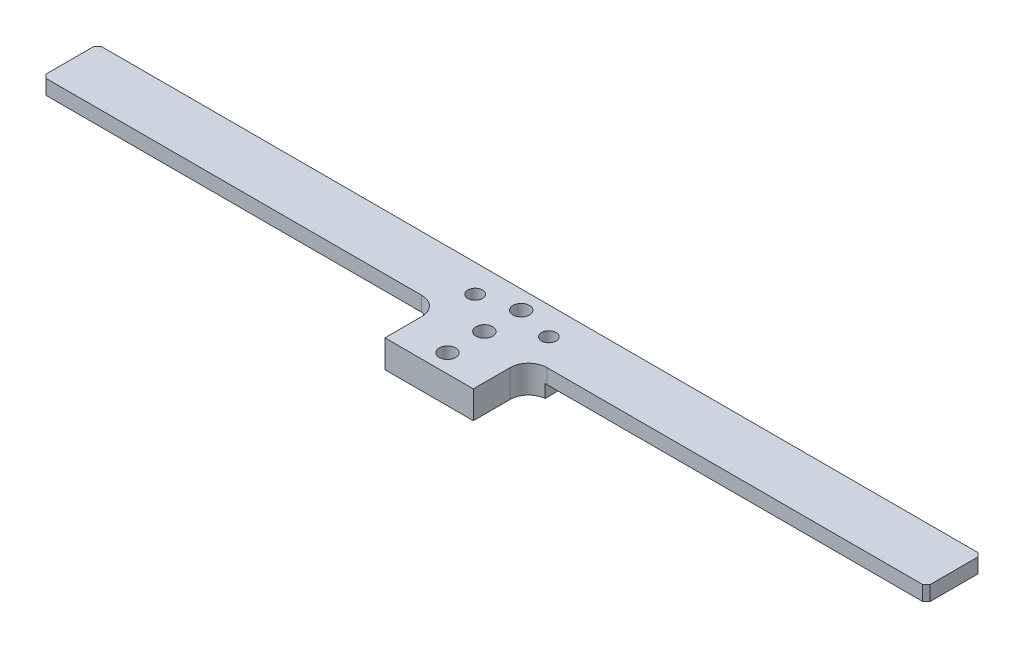
SolidWorks part; units mm, degrees
ref_plane "Front Plane" through (0, 0, 0) normal (0, 0, 1) x (1, 0, 0)
ref_plane "Top Plane" through (0, 0, 0) normal (0, 1, 0) x (1, 0, 0)
ref_plane "Right Plane" through (0, 0, 0) normal (1, 0, 0) x (0, 0, -1)
ref_plane "Plane 4" through (0, -2, 0) normal (0, -1, 0) x (1, 0, 0)
sketch "Sketch 1" plane through (0, -2, 0) normal (0, -1, 0) x (1, 0, 0)
  line L0 (-59, 15) -> (-69, 15)
  line L1 (-59, 15) -> (-58, 15)
  line L2 (-70, 15) -> (-70, -15)
  line L4 (-69, -15) -> (69, -15)
  line L5 (69, -15) -> (70, -14)
  line L6 (70, -14) -> (70, -1)
  line L7 (70, -1) -> (69, 0)
  line L8 (69, 0) -> (-53, 0)
  line L9 (-58, 5) -> (-58, 15)
  line L11 (-69, -15) -> (-70, -15)
  line L12 (-69, 15) -> (-70, 15)
  arc A3 (-53, 0) -> (-58, 5) centre (-53, 5) cw
  dimension "D1" = 5
extrude "Boss-Extrude 1" add sketch "Sketch 1" against normal blind 4
sketch "Sketch 2" plane through (0, 2, 0) normal (0, 1, 0) x (1, 0, 0)
  line L1 (-70, 15) -> (-190, 15)
  line L2 (-70, 15) -> (-70, -15)
  line L3 (-70, -15) -> (-82, -15)
  line L4 (-190, 15) -> (-190, 0)
  line L8 (-190, 0) -> (-82, 0)
  line L9 (-82, -15) -> (-82, 0)
  dimension "D1" = 120
  dimension "D2" = 12
  dimension "D3" = 15
extrude "Boss-Extrude 2" add sketch "Sketch 2" against normal blind 4
fillet "Fillet 1" radius 5 1 edges at (-82, 0, 0)
sketch "Sketch 6" plane through (0, -2, 0) normal (0, -1, 0) x (1, 0, 0)
  line L0 (-190, -15) -> (69, -15) construction
  line L1 (-82, 15) -> (-58, 15)
  line L2 (-82, 15) -> (-82, -15)
  line L3 (-82, -15) -> (-58, -15)
  line L4 (-58, 15) -> (-58, -15)
  dimension "D1" = 24
extrude "Boss-Extrude 3" add sketch "Sketch 6" along normal blind 3.5
sketch "Sketch 3" plane through (0, 2, 0) normal (0, 1, 0) x (1, 0, 0)
  line L0 (-82, -5) -> (-82, -15) construction
  line L2 (-58, -15) -> (-82, -15) construction
  circle A0 centre (-70, -10) radius 2.25
  dimension "D1" = 4.5
  dimension "D2" = 12
  dimension "D3" = 5
extrude "Cut-Extrude 1" cut sketch "Sketch 3" against normal through all
pattern_linear "Linear Pattern 1" count 3 spacing 10 along (0, 0, -1) of "Cut-Extrude 1"
sketch "Sketch 7" plane through (0, 2, 0) normal (0, 1, 0) x (1, 0, 0)
  line L0 (-58, -15) -> (-82, -15) construction
  line L1 (113.7784, -21.1495) -> (50, -21.1495)
  line L2 (113.7784, -21.1495) -> (113.7784, 35.093)
  line L3 (113.7784, 35.093) -> (50, 35.093)
  line L4 (50, -21.1495) -> (50, 35.093)
  point P6 (-70, -15)
  dimension "D1" = 120
extrude "Cut-Extrude 2" cut sketch "Sketch 7" against normal blind 10
chamfer "Chamfer 3" distance 1 angle 45 4 edges at (50, 0, -15) (50, 0, 0) (-190, 0, -15) (-190, 0, 0)
sketch "Sketch 8" plane through (0, -5.5, 0) normal (0, -1, 0) x (1, 0, 0)
  line L1 (-58, -15) -> (-53.5, -15)
  line L2 (-58, -15) -> (-58, 15)
  line L3 (-58, 15) -> (-53.5, 15)
  line L4 (-53.5, -15) -> (-53.5, 15)
  line L5 (-82, -15) -> (-86.5, -15)
  line L6 (-82, -15) -> (-82, 15)
  line L7 (-82, 15) -> (-86.5, 15)
  line L8 (-86.5, -15) -> (-86.5, 15)
  dimension "D1" = 30
  dimension "D2" = 4.5
  dimension "D3" = 4.5
  dimension "D4" = 30
extrude "Boss-Extrude 4" add sketch "Sketch 8" against normal up to surface (3.5 mm away) up to face at (-3.1429, -2, -7.5)
sketch "Sketch 9" plane through (0, -2, 0) normal (0, 1, 0) x (1, 0, 0)
  line L0 (-53.5, -15) -> (-58, -15)
  line L1 (-58, -15) -> (-58, -5)
  line L2 (-53.5, -15) -> (-53.5, -0.0251)
  line L3 (-82, -15) -> (-86.5, -15)
  line L4 (-86.5, -15) -> (-86.5, -0.0251)
  line L5 (-86.5, -15) -> (-86.5, -0.0251) construction
  line L6 (-82, -15) -> (-82, -5)
  arc A0 (-58, -5) -> (-53.5, -0.0251) centre (-53, -5) cw
  arc A1 (-86.5, -0.0251) -> (-82, -5) centre (-87, -5) cw
  arc A2 (-82, -5) -> (-86.5, -0.0251) centre (-87, -5) ccw construction
extrude "Cut-Extrude 3" cut sketch "Sketch 9" against normal blind 10
hole_wizard "Ø4.0 (4) Hole 1" positions "Sketch 11" profile "Sketch 10" hole size "Ø4.0" standard "JIS" end condition through all
sketch "Sketch 11" plane through (0, 2, 0) normal (0, 1, 0) x (-1, 0, 0)
  line L0 (189, -15) -> (-49, -15) construction
  line L2 (58, 15) -> (82, 15) construction
  point P0 (60, -7.5)
  point P8 (70, 15)
  dimension "D1" = 7.5
  dimension "D2" = 10
sketch "Sketch 10" plane through (-60, 2, -7.5) normal (1, 0, 0) x (0, 0, 1)
  line L0 (0, 0) -> (0, 7.5)
  line L1 (0, 7.5) -> (2, 7.5)
  line L2 (2, 7.5) -> (2, 0)
  line L5 (2, 0) -> (0, 0)
  line L11 (0, -6.35) -> (0, 107.95) construction
  dimension "貫穿孔直徑" = 4
  dimension "貫穿孔深度" = 7.5
pattern_linear "Linear Pattern 2" count 2 spacing 20 along (-1, 0, 0) of "Ø4.0 (4) Hole 1"
